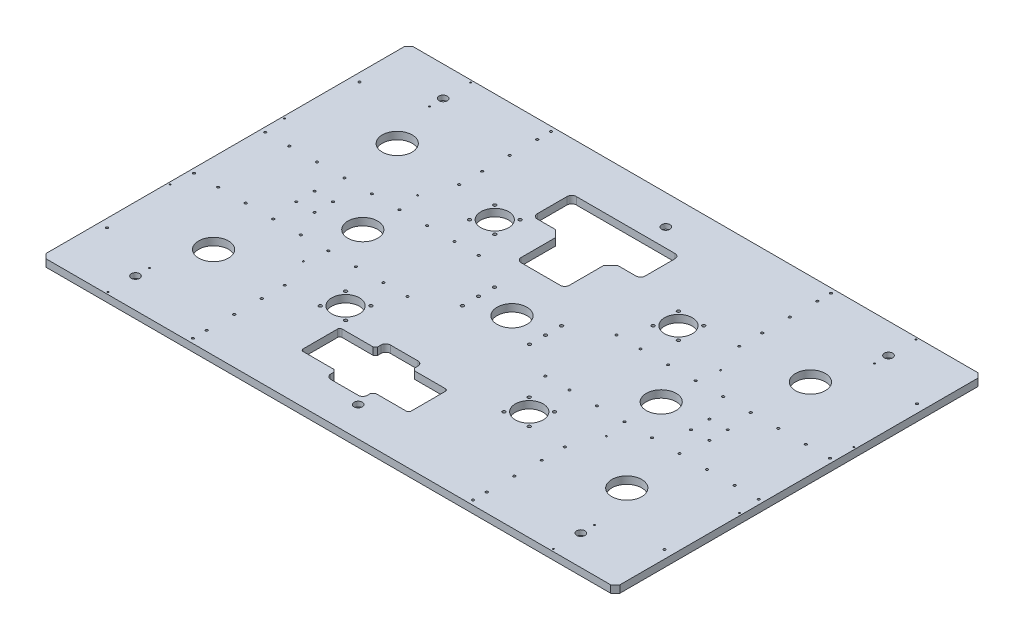
SolidWorks part; units mm, degrees
ref_plane "前视基准面" through (0, 0, 0) normal (0, 0, 1) x (1, 0, 0)
ref_plane "上视基准面" through (0, 0, 0) normal (0, 1, 0) x (1, 0, 0)
ref_plane "右视基准面" through (0, 0, 0) normal (1, 0, 0) x (0, 0, -1)
sketch "草图1" plane through (0, 0, 0) normal (0, 1, 0) x (1, 0, 0)
  line L1 (-625, 400) -> (625, 400)
  line L2 (-625, 400) -> (-625, -400)
  line L3 (-625, -400) -> (625, -400)
  line L4 (625, 400) -> (625, -400)
  line L5 (-625, 400) -> (625, -400) construction
  line L6 (-625, -400) -> (625, 400) construction
  point P0 (0, 0)
  dimension "D1" = 1250
  dimension "D2" = 800
extrude "凸台-拉伸1" add sketch "草图1" along normal mid plane 16
hole_wizard "M10 六角凹头螺钉的柱形沉头孔1" positions "草图3" profile "草图2" counterbore size "M10" standard "ISO" end condition through all
sketch "草图3" plane through (0, 8, 0) normal (0, 1, 0) x (1, 0, 0)
  point P0 (485, -335)
  point P2 (485, 335)
  dimension "D1" = 670
  dimension "D2" = 335
  dimension "D3" = 485
sketch "草图2" plane through (485, 8, 335) normal (1, 0, 0) x (0, 0, 1)
  line L0 (0, 0) -> (0, 16)
  line L1 (0, 16) -> (5.5, 16)
  line L3 (5.5, 16) -> (5.5, 10.6)
  line L4 (5.5, 10.6) -> (9, 10.6)
  line L5 (9, 10.6) -> (9, 0)
  line L7 (9, 0) -> (0, 0)
  line L11 (0, -6.35) -> (0, 107.95) construction
  dimension "通孔孔直径" = 11
  dimension "通孔孔深度" = 16
  dimension "柱形沉头孔直径" = 18
  dimension "柱形沉头孔深度" = 10.6
sketch "草图4" plane through (0, 8, 0) normal (0, 1, 0) x (1, 0, 0)
  line L0 (-625, -400) -> (625, -400) construction
  line L1 (-160, -210) -> (-92.5, -210)
  line L2 (-165, -215) -> (-165, -290)
  line L3 (-160, -295) -> (-92.5, -295)
  line L4 (70, -215) -> (70, -290)
  line L5 (-165, -210) -> (70, -295) construction
  line L6 (-165, -295) -> (70, -210) construction
  line L7 (-47.5, -166.3452) -> (-47.5, -352.1496) construction
  line L8 (-7.5, -300) -> (-7.5, -307.5)
  line L9 (-77.5, -187.5) -> (-17.5, -187.5)
  line L10 (-87.5, -197.5) -> (-87.5, -205)
  line L11 (-77.5, -317.5) -> (-17.5, -317.5)
  line L12 (-7.5, -197.5) -> (-7.5, -205)
  line L13 (-87.5, -187.5) -> (-7.5, -317.5) construction
  line L14 (-87.5, -317.5) -> (-7.5, -187.5) construction
  line L15 (-87.5, -300) -> (-87.5, -307.5)
  line L16 (-2.5, -295) -> (65, -295)
  line L17 (-2.5, -210) -> (65, -210)
  line L18 (0, 435.3406) -> (0, -588.1926) construction
  line L19 (0, -79.6524) -> (0, 79.6524) construction
  line L20 (-92.5, -210) -> (-87.5, -205)
  line L21 (-7.5, -205) -> (-2.5, -210)
  line L22 (-7.5, -300) -> (-2.5, -295)
  line L23 (-92.5, -295) -> (-87.5, -300)
  arc A1 (-87.5, -307.5) -> (-77.5, -317.5) centre (-77.5, -307.5) ccw
  arc A2 (-17.5, -317.5) -> (-7.5, -307.5) centre (-17.5, -307.5) ccw
  arc A3 (-7.5, -197.5) -> (-17.5, -187.5) centre (-17.5, -197.5) ccw
  arc A4 (-77.5, -187.5) -> (-87.5, -197.5) centre (-77.5, -197.5) ccw
  arc A9 (65, -210) -> (70, -215) centre (65, -215) cw
  arc A10 (70, -290) -> (65, -295) centre (65, -290) cw
  arc A11 (-165, -290) -> (-160, -295) centre (-160, -290) ccw
  arc A12 (-165, -215) -> (-160, -210) centre (-160, -215) cw
  point P0 (-47.5, -252.5)
  point P10 (-47.5, -252.5)
  point P11 (-47.5, -252.5)
  point P33 (-7.5, -210)
  point P38 (-7.5, -295)
  point P59 (-87.5, -210)
  point P62 (-7.5, -295)
  point P65 (-87.5, -295)
  dimension "D7" = 10
  dimension "D9" = 5
  dimension "D1" = 235
  dimension "D2" = 85
  dimension "D3" = 165
  dimension "D4" = 105
  dimension "D5" = 80
  dimension "D6" = 130
  dimension "D10" = 47.5
extrude "切除-拉伸1" cut sketch "草图4" against normal blind 16
sketch "草图5" plane through (0, 8, 0) normal (0, 1, 0) x (1, 0, 0)
  line L0 (625, 400) -> (-625, 400) construction
  line L1 (-155, 295) -> (60, 295)
  line L2 (-165, 285) -> (-165, 220)
  line L3 (-155, 210) -> (-115, 210)
  line L4 (70, 285) -> (70, 220)
  line L5 (-47.5, 332.0626) -> (-47.5, 19.4592) construction
  line L6 (20, 210) -> (60, 210)
  line L7 (-115, 210) -> (-100, 195)
  line L8 (-100, 195) -> (-100, 120)
  line L9 (-90, 110) -> (-5, 110)
  line L10 (5, 195) -> (5, 120)
  line L11 (5, 195) -> (20, 210)
  arc A0 (60, 295) -> (70, 285) centre (60, 285) cw
  arc A1 (70, 220) -> (60, 210) centre (60, 220) cw
  arc A2 (-100, 120) -> (-90, 110) centre (-90, 120) ccw
  arc A3 (-5, 110) -> (5, 120) centre (-5, 120) ccw
  arc A5 (-165, 220) -> (-155, 210) centre (-155, 220) ccw
  arc A6 (-155, 295) -> (-165, 285) centre (-155, 285) ccw
  point P9 (-100, 210)
  point P15 (70, 295)
  point P18 (70, 210)
  point P21 (-100, 110)
  point P24 (5, 110)
  point P31 (-165, 295)
  point P36 (5, 210)
  dimension "D8" = 10
  dimension "D1" = 235
  dimension "D2" = 85
  dimension "D3" = 165
  dimension "D4" = 105
  dimension "D5" = 100
  dimension "D6" = 105
  dimension "D7" = 52.5
extrude "切除-拉伸2" cut sketch "草图5" against normal blind 16
sketch "草图6" plane through (0, 8, 0) normal (0, 1, 0) x (1, 0, 0)
  line L0 (0, 116.1277) -> (0, -190.1984) construction
  circle A0 centre (450, 200) radius 32.5
  circle A1 centre (325, 0) radius 32.5
  circle A2 centre (450, -200) radius 32.5
  circle A3 centre (0, 0) radius 32.5
  circle A4 centre (-450, -200) radius 32.5
  circle A5 centre (-325, 0) radius 32.5
  circle A6 centre (-450, 200) radius 32.5
  dimension "D1" = 65
  dimension "D2" = 65
  dimension "D3" = 65
  dimension "D5" = 200
  dimension "D6" = 450
  dimension "D8" = 65
  dimension "D4" = 400
  dimension "D7" = 325
extrude "切除-拉伸3" cut sketch "草图6" against normal blind 16
sketch "草图7" plane through (0, 8, 0) normal (0, 1, 0) x (1, 0, 0)
  circle A0 centre (200, -162.5) radius 30.25
  dimension "D1" = 60.5
  dimension "D3" = 162.5
  dimension "D2" = 200
extrude "切除-拉伸4" cut sketch "草图7" against normal blind 16
hole_wizard "M8 螺纹孔1" positions "草图9" profile "草图8" tap size "M8" standard "ISO"
sketch "草图9" plane through (0, 8, 0) normal (0, 1, 0) x (1, 0, 0)
  line L0 (200, -222.8492) -> (200, -97.7295) construction
  line L2 (200, -162.5) -> (141.993, -104.493) construction
  circle A0 centre (200, -162.5) radius 39 construction
  point P13 (172.4228, -134.9228)
  point P26 (227.5772, -134.9228)
  point P27 (227.5772, -190.0772)
  point P28 (172.4228, -190.0772)
  point P29 (200, -162.5)
  dimension "D1" = 78
  dimension "D2" = 45
  dimension "D3" = 4
sketch "草图8" plane through (172.4228, 8, 134.9228) normal (1, 0, 0) x (0, 0, 1)
  line L0 (0, 0) -> (0, 16)
  line L1 (0, 16) -> (3.4, 16)
  line L2 (3.4, 16) -> (3.4, 0)
  line L5 (3.4, 0) -> (0, 0)
  line L11 (0, -6.35) -> (0, 107.95) construction
  dimension "通孔螺纹孔钻头直径" = 6.8
  dimension "通孔螺纹孔钻头深度" = 16
cosmetic thread "孔螺蚊线1" parameters "D2"=8
cosmetic thread "孔螺蚊线2" parameters "D2"=8
cosmetic thread "孔螺蚊线3" parameters "D2"=8
cosmetic thread "孔螺蚊线4" parameters "D2"=8
pattern_linear "阵列(线性)2" count 2 spacing 400 along (-1, 0, 0) of "M8 螺纹孔1"
pattern_linear "阵列(线性)3" count 2 spacing 325 along (0, 0, -1) of "阵列(线性)2", "M8 螺纹孔1"
mirror "镜向5" about plane through (0, 0, 0) normal (0, 0, 1) of "切除-拉伸4"
mirror "镜向6" about plane through (0, 0, 0) normal (1, 0, 0) of "切除-拉伸4", "镜向5"
pattern_linear "阵列(线性)10" count 3 spacing 485 along (-1, 0, 0) of "M10 六角凹头螺钉的柱形沉头孔1"
hole_wizard "M6 螺纹孔2" positions "草图16" profile "草图15" tap size "M6" standard "ISO"
sketch "草图16" plane through (0, 8, 0) normal (0, 1, 0) x (1, 0, 0)
  line L0 (-625, 400) -> (-625, -400) construction
  point P0 (-607, 275)
  dimension "D1" = 18
  dimension "D2" = 275
cosmetic thread "孔螺蚊线141" parameters "D2"=6
sketch "草图15" plane through (-607, 8, -275) normal (1, 0, 0) x (0, 0, 1)
  line L0 (0, 0) -> (0, 16)
  line L1 (0, 16) -> (2.5, 16)
  line L2 (2.5, 16) -> (2.5, 0)
  line L5 (2.5, 0) -> (0, 0)
  line L11 (0, -6.35) -> (0, 107.95) construction
  dimension "通孔螺纹孔钻头直径" = 5
  dimension "通孔螺纹孔钻头深度" = 16
mirror "镜向7" about plane through (0, 0, 0) normal (0, 0, 1) of "M6 螺纹孔2"
mirror "镜向8" about plane through (0, 0, 0) normal (1, 0, 0) of "镜向7", "M6 螺纹孔2"
hole_wizard "M6 螺纹孔1" positions "草图18" profile "草图17" tap size "M6" standard "ISO"
sketch "草图18" plane through (0, 8, 0) normal (0, 1, 0) x (1, 0, 0)
  line L0 (-625, 400) -> (-625, -400) construction
  point P0 (-450, 20)
  point P3 (-625, 0)
  dimension "D1" = 175
  dimension "D2" = 20
sketch "草图17" plane through (-450, 8, -20) normal (1, 0, 0) x (0, 0, 1)
  line L0 (0, 0) -> (0, 16)
  line L1 (0, 16) -> (2.5, 16)
  line L2 (2.5, 16) -> (2.5, 0)
  line L5 (2.5, 0) -> (0, 0)
  line L11 (0, -6.35) -> (0, 107.95) construction
  dimension "通孔螺纹孔钻头直径" = 5
  dimension "通孔螺纹孔钻头深度" = 16
cosmetic thread "孔螺蚊线142" parameters "D2"=6
mirror "镜向9" about plane through (0, 0, 0) normal (0, 0, 1) of "M6 螺纹孔1"
pattern_linear "阵列(线性)11" count 2 spacing 40 along (1, 0, 0) of "镜向9", "M6 螺纹孔1"
mirror "镜向10" about plane through (0, 0, 0) normal (1, 0, 0) of "阵列(线性)11", "M6 螺纹孔1", "镜向9"
hole_wizard "M8 螺纹孔5" positions "草图20" profile "草图19" tap size "M8" standard "ISO"
sketch "草图20" plane through (0, 8, 0) normal (0, 1, 0) x (1, 0, 0)
  point P0 (-73, -35)
  dimension "D1" = 73
  dimension "D2" = 35
sketch "草图19" plane through (-73, 8, 35) normal (1, 0, 0) x (0, 0, 1)
  line L0 (0, 0) -> (0, 16)
  line L1 (0, 16) -> (3.4, 16)
  line L2 (3.4, 16) -> (3.4, 0)
  line L5 (3.4, 0) -> (0, 0)
  line L11 (0, -6.35) -> (0, 107.95) construction
  dimension "通孔螺纹孔钻头直径" = 6.8
  dimension "通孔螺纹孔钻头深度" = 16
cosmetic thread "孔螺蚊线143" parameters "D2"=8
pattern_linear "阵列(线性)12" count 3 spacing 35 along (0, 0, -1) of "M8 螺纹孔5"
mirror "镜向11" about plane through (0, 0, 0) normal (1, 0, 0) of "阵列(线性)12", "M8 螺纹孔5"
chamfer "倒角1" distance 10 angle 45 4 edges at (-625, 0, -400) (625, 0, -400) (625, 0, 400) (-625, 0, 400)
hole_wizard "M6 螺纹孔3" positions "草图22" profile "草图21" tap size "M6" standard "ISO"
sketch "草图22" plane through (0, 8, 0) normal (0, 1, 0) x (1, 0, 0)
  point P0 (-305, 190)
  point P3 (-305, 390)
  point P6 (-305, 360)
  point P9 (-305, 300)
  point P12 (-305, 240)
sketch "草图21" plane through (-305, 8, -190) normal (1, 0, 0) x (0, 0, 1)
  line L0 (0, 0) -> (0, 16)
  line L1 (0, 16) -> (2.5, 16)
  line L2 (2.5, 16) -> (2.5, 0)
  line L5 (2.5, 0) -> (0, 0)
  line L11 (0, -6.35) -> (0, 107.95) construction
  dimension "通孔螺纹孔钻头直径" = 5
  dimension "通孔螺纹孔钻头深度" = 16
cosmetic thread "孔螺蚊线144" parameters "D2"=6
cosmetic thread "孔螺蚊线145" parameters "D2"=6
cosmetic thread "孔螺蚊线146" parameters "D2"=6
cosmetic thread "孔螺蚊线147" parameters "D2"=6
cosmetic thread "孔螺蚊线148" parameters "D2"=6
hole_wizard "M6 螺纹孔4" positions "草图24" profile "草图23" tap size "M6" standard "ISO"
sketch "草图24" plane through (0, 8, 0) normal (0, 1, 0) x (1, 0, 0)
  point P0 (-150, -77.5)
  point P3 (-202.5, -77.5)
  point P6 (-262.5, -77.5)
  point P9 (-322.5, -77.5)
  point P12 (-382.5, -77.5)
  point P15 (-442.5, -77.5)
  point P18 (-502.5, -77.5)
  point P21 (-562.5, -77.5)
  point P24 (-615, -77.5)
sketch "草图23" plane through (-150, 8, 77.5) normal (1, 0, 0) x (0, 0, 1)
  line L0 (0, 0) -> (0, 16)
  line L1 (0, 16) -> (2.5, 16)
  line L2 (2.5, 16) -> (2.5, 0)
  line L5 (2.5, 0) -> (0, 0)
  line L11 (0, -6.35) -> (0, 107.95) construction
  dimension "通孔螺纹孔钻头直径" = 5
  dimension "通孔螺纹孔钻头深度" = 16
cosmetic thread "孔螺蚊线149" parameters "D2"=6
cosmetic thread "孔螺蚊线150" parameters "D2"=6
cosmetic thread "孔螺蚊线151" parameters "D2"=6
cosmetic thread "孔螺蚊线152" parameters "D2"=6
cosmetic thread "孔螺蚊线153" parameters "D2"=6
cosmetic thread "孔螺蚊线154" parameters "D2"=6
cosmetic thread "孔螺蚊线155" parameters "D2"=6
cosmetic thread "孔螺蚊线156" parameters "D2"=6
cosmetic thread "孔螺蚊线157" parameters "D2"=6
ref_plane "基准面1" through (0, 0, 0) normal (0, 0, 1) x (1, 0, 0)
mirror "镜向12" about plane through (0, 0, 0) normal (0, 0, 1) of "M6 螺纹孔3", "M6 螺纹孔4"
ref_plane "基准面2" through (0, 0, 0) normal (-1, 0, 0) x (0, 0, 1)
mirror "镜向13" about plane through (0, 0, 0) normal (-1, 0, 0) of "镜向12", "M6 螺纹孔4", "M6 螺纹孔3"
hole_wizard "M4 螺纹孔1" positions "草图26" profile "草图25" tap size "M4" standard "ISO"
sketch "草图26" plane through (0, 8, 0) normal (0, 1, 0) x (1, 0, 0)
  point P0 (-620, -124.5)
  point P3 (-620, 124.5)
  point P6 (-330, 124.5)
  point P9 (-330, -124.5)
sketch "草图25" plane through (-620, 8, 124.5) normal (1, 0, 0) x (0, 0, 1)
  line L0 (0, 0) -> (0, 16)
  line L1 (0, 16) -> (1.65, 16)
  line L2 (1.65, 16) -> (1.65, 0)
  line L5 (1.65, 0) -> (0, 0)
  line L11 (0, -6.35) -> (0, 107.95) construction
  dimension "通孔螺纹孔钻头直径" = 3.3
  dimension "通孔螺纹孔钻头深度" = 16
cosmetic thread "孔螺蚊线158" parameters "D2"=4
cosmetic thread "孔螺蚊线159" parameters "D2"=4
cosmetic thread "孔螺蚊线160" parameters "D2"=4
cosmetic thread "孔螺蚊线161" parameters "D2"=4
hole_wizard "M4 螺纹孔2" positions "草图28" profile "草图27" tap size "M4" standard "ISO"
sketch "草图28" plane through (0, 8, 0) normal (0, 1, 0) x (1, 0, 0)
  point P0 (330, -124.5)
  point P3 (620, -124.5)
  point P6 (620, 124.5)
  point P9 (330, 124.5)
sketch "草图27" plane through (330, 8, 124.5) normal (1, 0, 0) x (0, 0, 1)
  line L0 (0, 0) -> (0, 16)
  line L1 (0, 16) -> (1.65, 16)
  line L2 (1.65, 16) -> (1.65, 0)
  line L5 (1.65, 0) -> (0, 0)
  line L11 (0, -6.35) -> (0, 107.95) construction
  dimension "通孔螺纹孔钻头直径" = 3.3
  dimension "通孔螺纹孔钻头深度" = 16
cosmetic thread "孔螺蚊线162" parameters "D2"=4
cosmetic thread "孔螺蚊线163" parameters "D2"=4
cosmetic thread "孔螺蚊线164" parameters "D2"=4
cosmetic thread "孔螺蚊线165" parameters "D2"=4
hole_wizard "M4 螺纹孔3" positions "草图30" profile "草图29" tap size "M4" standard "ISO"
sketch "草图30" plane through (0, 8, 0) normal (0, 1, 0) x (1, 0, 0)
  point P0 (-484.8781, 305)
  point P3 (-484.8781, 395)
sketch "草图29" plane through (-484.8781, 8, -305) normal (1, 0, 0) x (0, 0, 1)
  line L0 (0, 0) -> (0, 16)
  line L1 (0, 16) -> (1.65, 16)
  line L2 (1.65, 16) -> (1.65, 0)
  line L5 (1.65, 0) -> (0, 0)
  line L11 (0, -6.35) -> (0, 107.95) construction
  dimension "通孔螺纹孔钻头直径" = 3.3
  dimension "通孔螺纹孔钻头深度" = 16
cosmetic thread "孔螺蚊线166" parameters "D2"=4
cosmetic thread "孔螺蚊线167" parameters "D2"=4
mirror "镜向14" about plane through (0, 0, 0) normal (-1, 0, 0) of "M4 螺纹孔3"
mirror "镜向15" about plane through (0, 0, 0) normal (0, 0, 1) of "镜向14", "M4 螺纹孔3"
